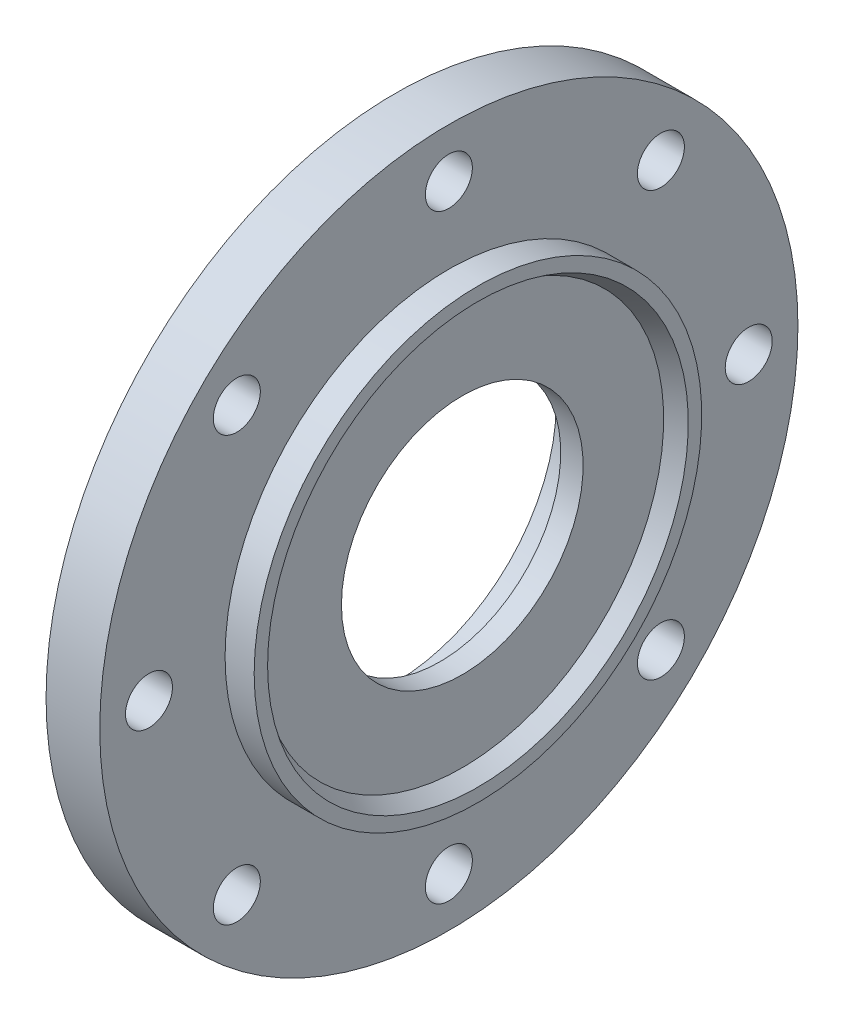
from build123d import *

# Parameters (mm, degrees)
SKETCH2_R          = 5.25
CUT_EXTRUDE1_DEPTH = 112.849228875
CIRPATTERN1_COUNT  = 8


with BuildPart() as part:
    # Sketch1 → Revolve1 (revolve)
    with BuildSketch(Plane.XY, mode=Mode.PRIVATE) as revolve1_sk:
        Polygon((0, 36), (0, 78), (12, 78), (12, 50), (18.5, 50), (18.5, 47), (15, 45), (15, 27), (10, 27), (10, 36), align=None)
    revolve(revolve1_sk.sketch.rotate(Axis((0, 0, 0), (1, 0, 0)), 90), axis=Axis((0, 0, 0), (1, 0, 0)))

    # Sketch2 → Cut-Extrude1 (cut, through all)
    with BuildSketch(Plane.ZY):
        with Locations((0, 67)):
            Circle(SKETCH2_R)
    cut_extrude1 = extrude(amount=-CUT_EXTRUDE1_DEPTH, mode=Mode.SUBTRACT)

    # CirPattern1: Cut-Extrude1 ×8 about axis
    cirpattern1_axis = Axis((0, 0, 0), (1, 0, 0))
    for i in range(1, CIRPATTERN1_COUNT):
        add(cut_extrude1.rotate(cirpattern1_axis, i * 360 / CIRPATTERN1_COUNT), mode=Mode.SUBTRACT)


solid = part.part
